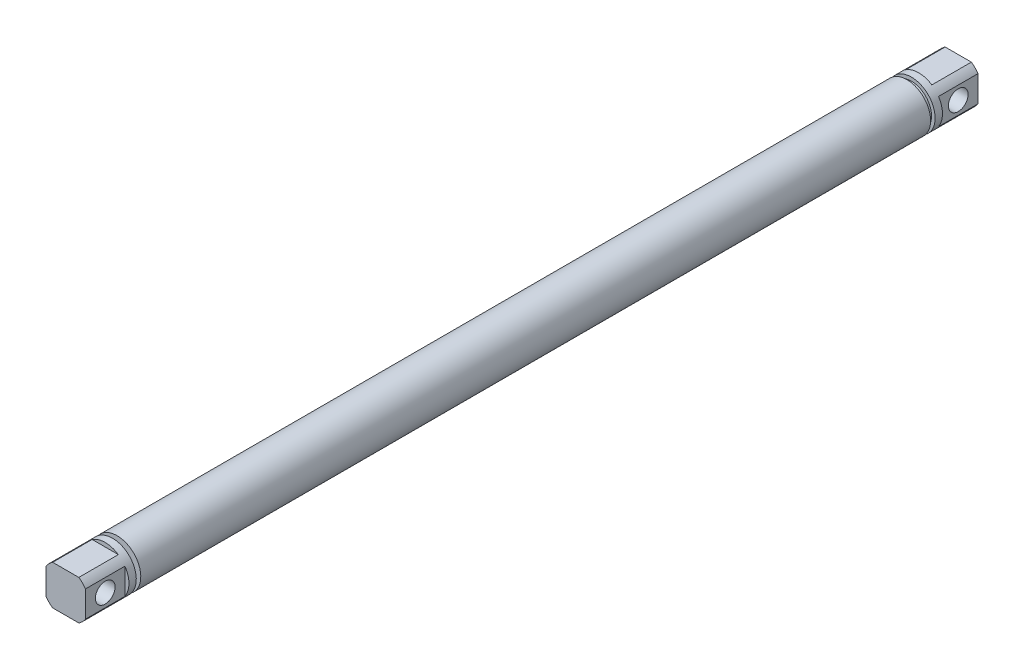
from build123d import *

# Parameters (mm, degrees)
SKETCH_1_R          = 6
EXTRUDE_1_DEPTH     = 113
SKETCH_2_W          = 1.14
SKETCH_2_H          = 0.9
SKETCH_2_H_2        = 1.654271951
CUT_EXTRUDE_START   = -10
CUT_EXTRUDE_1_DEPTH = 10
HOLE_WIZARD_M6_1_D  = 5


with BuildPart() as part:
    # 草图1 → 凸台-拉伸1 (new, symmetric)
    with BuildSketch(Plane.XY):
        Circle(SKETCH_1_R)
    extrude(amount=EXTRUDE_1_DEPTH, both=True)

    # 草图2 → 切除-旋转1 (revolve, cut)
    with BuildSketch(Plane(origin=(0, 0, 0), x_dir=(0, 0, -1), z_dir=(1, 0, 0)), mode=Mode.PRIVATE) as cut_revolve_1_sk:
        with Locations((100.57, 5.55)):
            Rectangle(SKETCH_2_W, SKETCH_2_H)
        with Locations((-100.57, 5.172864024)):
            Rectangle(SKETCH_2_W, SKETCH_2_H_2)
    revolve(cut_revolve_1_sk.sketch.rotate(Axis((0, 0, 0), (0, 0, -1)), 180), axis=Axis((0, 0, 0), (0, 0, -1)), mode=Mode.SUBTRACT)

    # 草图3 → 切除-拉伸1 (cut)
    with BuildSketch(Plane(origin=(0, 0, -113), x_dir=(-1, 0, 0), z_dir=(0, 0, -1)).offset(CUT_EXTRUDE_START)):
        with BuildLine():
            Line((-5, 3.31662479), (-5, -3.31662479))
            ThreePointArc((-5, -3.31662479), (-6, 0), (-5, 3.31662479))
        make_face()
        with BuildLine():
            Line((5, 3.31662479), (5, -3.31662479))
            ThreePointArc((5, -3.31662479), (6, 0), (5, 3.31662479))
        make_face()
        with BuildLine():
            Line((-3.31662479, 5), (3.31662479, 5))
            ThreePointArc((3.31662479, 5), (0, 6), (-3.31662479, 5))
        make_face()
        with BuildLine():
            Line((3.31662479, -5), (-3.31662479, -5))
            ThreePointArc((-3.31662479, -5), (0, -6), (3.31662479, -5))
        make_face()
    cut_extrude_1 = extrude(amount=CUT_EXTRUDE_1_DEPTH, mode=Mode.SUBTRACT)

    # M6 螺纹孔1 (through all)
    with Locations(Plane.ZY.offset(5)):
        with Locations((-108, 0)):
            hole_wizard_m6_1 = Hole(HOLE_WIZARD_M6_1_D / 2)

    # 镜向1: 切除-拉伸1, M6 螺纹孔1 across plane
    add(cut_extrude_1.mirror(Plane.XY), mode=Mode.SUBTRACT)
    add(hole_wizard_m6_1.mirror(Plane.XY), mode=Mode.SUBTRACT)


solid = part.part
